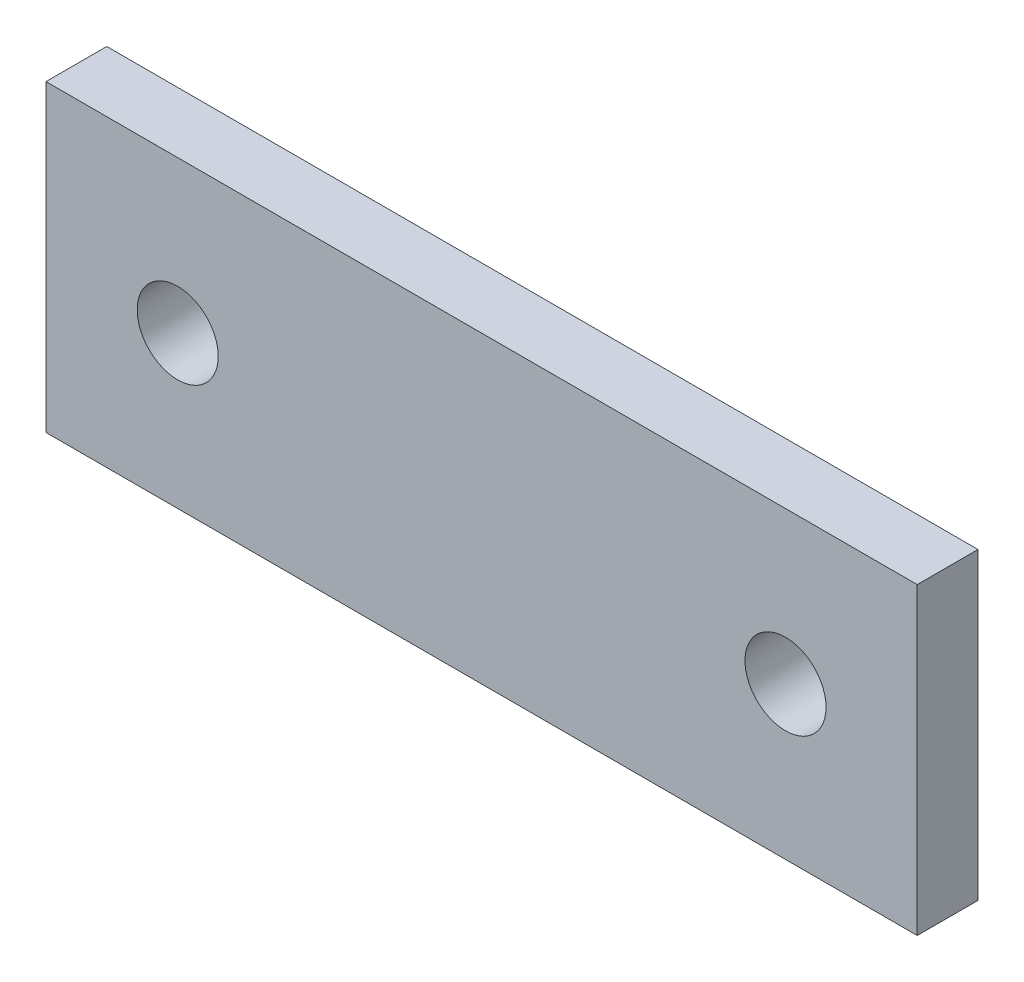
SolidWorks part; units mm, degrees
material "1023 Carbon Steel Plate (SS)"
ref_plane "Front Plane" through (0, 0, 0) normal (0, 0, 1) x (1, 0, 0)
ref_plane "Top Plane" through (0, 0, 0) normal (0, 1, 0) x (1, 0, 0)
ref_plane "Right Plane" through (0, 0, 0) normal (1, 0, 0) x (0, 0, -1)
sketch "Sketch1" plane through (0, 0, 0) normal (0, 0, 1) x (1, 0, 0)
  line L1 (43, 15) -> (-43, 15)
  line L2 (43, 15) -> (43, -15)
  line L3 (43, -15) -> (-43, -15)
  line L4 (-43, 15) -> (-43, -15)
  line L5 (43, 15) -> (-43, -15) construction
  line L6 (43, -15) -> (-43, 15) construction
  point P0 (0, 0)
  dimension "D1" = 86
  dimension "D2" = 30
extrude "Boss-Extrude1" add sketch "Sketch1" along normal blind 6
sketch "Sketch2" plane through (0, 0, 6) normal (0, 0, 1) x (1, 0, 0)
  circle A0 centre (-30, 0) radius 4
  circle A1 centre (30, 0) radius 4
  dimension "D1" = 8
  dimension "D2" = 8
  dimension "D3" = 60
  dimension "D4" = 30
extrude "Cut-Extrude1" cut sketch "Sketch2" against normal blind 10
